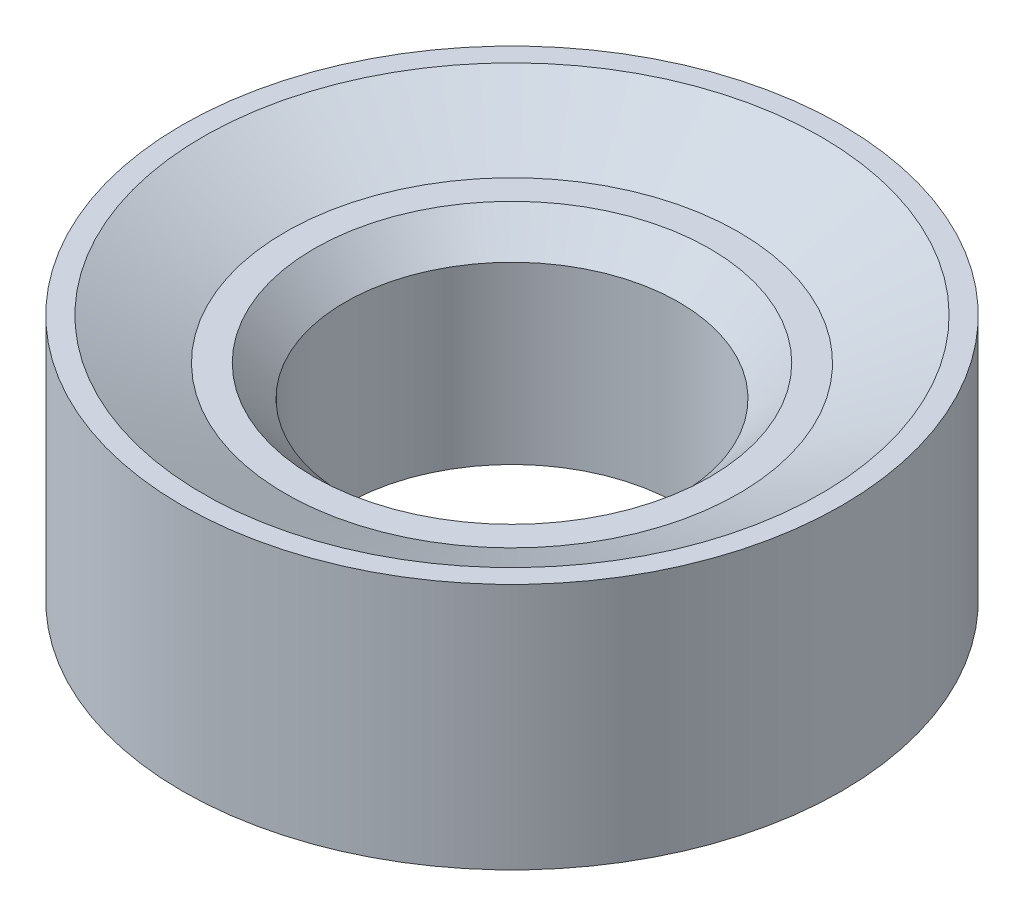
from build123d import *

# Parameters (mm, degrees)
M42X1_5_TAPPED_HOLE1_D     = 40.5
M42X1_5_TAPPED_HOLE1_DEPTH = 88.5
M42X1_5_TAPPED_HOLE1_TIP   = 12.167427535


with BuildPart() as part:
    # Sketch1 → Revolve1 (revolve)
    with BuildSketch(Plane.XY, mode=Mode.PRIVATE) as revolve1_sk:
        Polygon((20, 0), (40, 0), (40, 30), (37.5, 30), (27.5, 25), (24, 25), (20, 21), align=None)
    revolve(revolve1_sk.sketch.rotate(Axis((0, 0, 0), (0, 1, 0)), 90), axis=Axis((0, 0, 0), (0, 1, 0)))

    # M42X1.5 Tapped Hole1
    with Locations(Plane(origin=(0, 0, 0), x_dir=(-1, 0, 0), z_dir=(0, -1, 0))):
        with Locations((0, 0)):
            Hole(M42X1_5_TAPPED_HOLE1_D / 2, depth=M42X1_5_TAPPED_HOLE1_DEPTH)
            with Locations((0, 0, -(M42X1_5_TAPPED_HOLE1_DEPTH + M42X1_5_TAPPED_HOLE1_TIP / 2))):  # 118° drill point
                Cone(0, M42X1_5_TAPPED_HOLE1_D / 2, M42X1_5_TAPPED_HOLE1_TIP, mode=Mode.SUBTRACT)


solid = part.part
